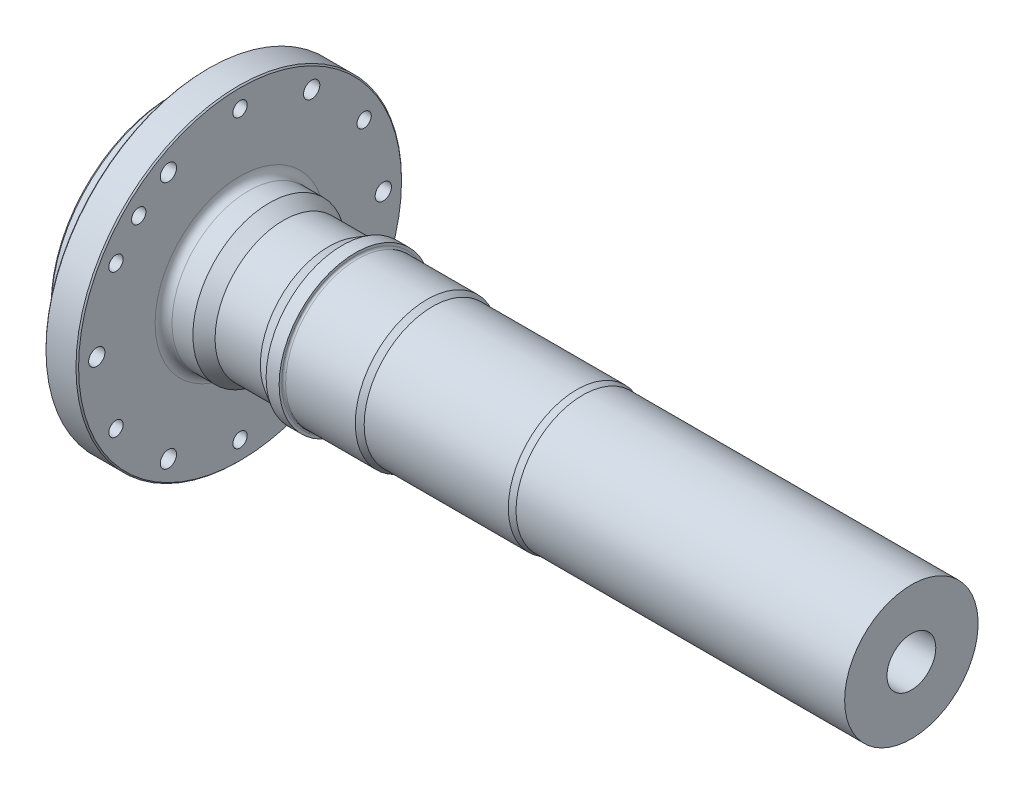
from build123d import *

# Parameters (mm, degrees)
M24X2_0_TAPPED_HOLE1_D = 22
SKETCH2_R              = 12.5
CUT_EXTRUDE1_DEPTH     = 1138.348231634
SKETCH4_R              = 37.5
CUT_EXTRUDE2_DEPTH     = 1190.746191421


with BuildPart() as part:
    # Sketch1 → Revolve1 (revolve)
    with BuildSketch(Plane.XY, mode=Mode.PRIVATE) as revolve1_sk:
        with BuildLine():
            Line((0, 0), (0, 185))
            Line((0, 185), (5, 190))
            Line((5, 190), (47, 190))
            Line((47, 190), (47.8, 189.2))
            Line((47.8, 189.2), (53.8, 189.2))
            ThreePointArc((53.8, 189.2), (55.214213562, 189.785786438), (55.8, 191.2))
            Line((55.8, 191.2), (55.8, 197.2))
            Line((55.8, 197.2), (55, 198))
            Line((55, 198), (55, 248))
            Line((55, 248), (57, 250))
            Line((57, 250), (103, 250))
            Line((103, 250), (105, 248))
            Line((105, 248), (105, 130.475))
            ThreePointArc((105, 130.475), (108.807611845, 121.282611845), (118, 117.475))
            Line((118, 117.475), (150, 117.475))
            Line((150, 117.475), (171.607333824, 105))
            Line((171.607333824, 105), (241.215390309, 105))
            Line((241.215390309, 105), (262, 117))
            Line((262, 117), (282, 117))
            Line((282, 117), (282, 113))
            ThreePointArc((282, 113), (282.878679656, 110.878679656), (285, 110))
            Line((285, 110), (392, 110))
            Line((392, 110), (400.660254038, 105))
            Line((400.660254038, 105), (622, 105))
            Line((622, 105), (631.330127019, 102.5))
            Line((631.330127019, 102.5), (1136, 102.5))
            Line((1136, 102.5), (1136, 0))
            Line((1136, 0), (0, 0))
        make_face()
    revolve(revolve1_sk.sketch.rotate(Axis((0, 0, 0), (1, 0, 0)), 90), axis=Axis((0, 0, 0), (1, 0, 0)))

    # M24x2.0 Tapped Hole1 (through all)
    with Locations(Plane(origin=(55, 220, 0), x_dir=(0, 0, -1), z_dir=(-1, 0, 0))):
        with Locations((0, 0), (-190.525588833, 110), (190.525588833, 110), (190.525588833, 330), (0, 440), (-190.525588833, 330), (-155.563491861, 64.436508139), (155.563491861, 375.563491861)):
            Hole(M24X2_0_TAPPED_HOLE1_D / 2)

    # Sketch2 → Cut-Extrude1 (cut, through all)
    with BuildSketch(Plane.ZY.offset(-55)):
        with Locations((-110, 190.525588833)):
            Circle(SKETCH2_R)
        with Locations((110, 190.525588833)):
            Circle(SKETCH2_R)
        with Locations((220, 0)):
            Circle(SKETCH2_R)
        with Locations((110, -190.525588833)):
            Circle(SKETCH2_R)
        with Locations((-110, -190.525588833)):
            Circle(SKETCH2_R)
        with Locations((-220, 0)):
            Circle(SKETCH2_R)
    extrude(amount=-CUT_EXTRUDE1_DEPTH, mode=Mode.SUBTRACT)

    # Sketch4 → Cut-Extrude2 (cut, through all)
    with BuildSketch(Plane(origin=(1136, 0, 0), x_dir=(0, 0, -1), z_dir=(1, 0, 0))):
        Circle(SKETCH4_R)
    extrude(amount=-CUT_EXTRUDE2_DEPTH, mode=Mode.SUBTRACT)


solid = part.part
